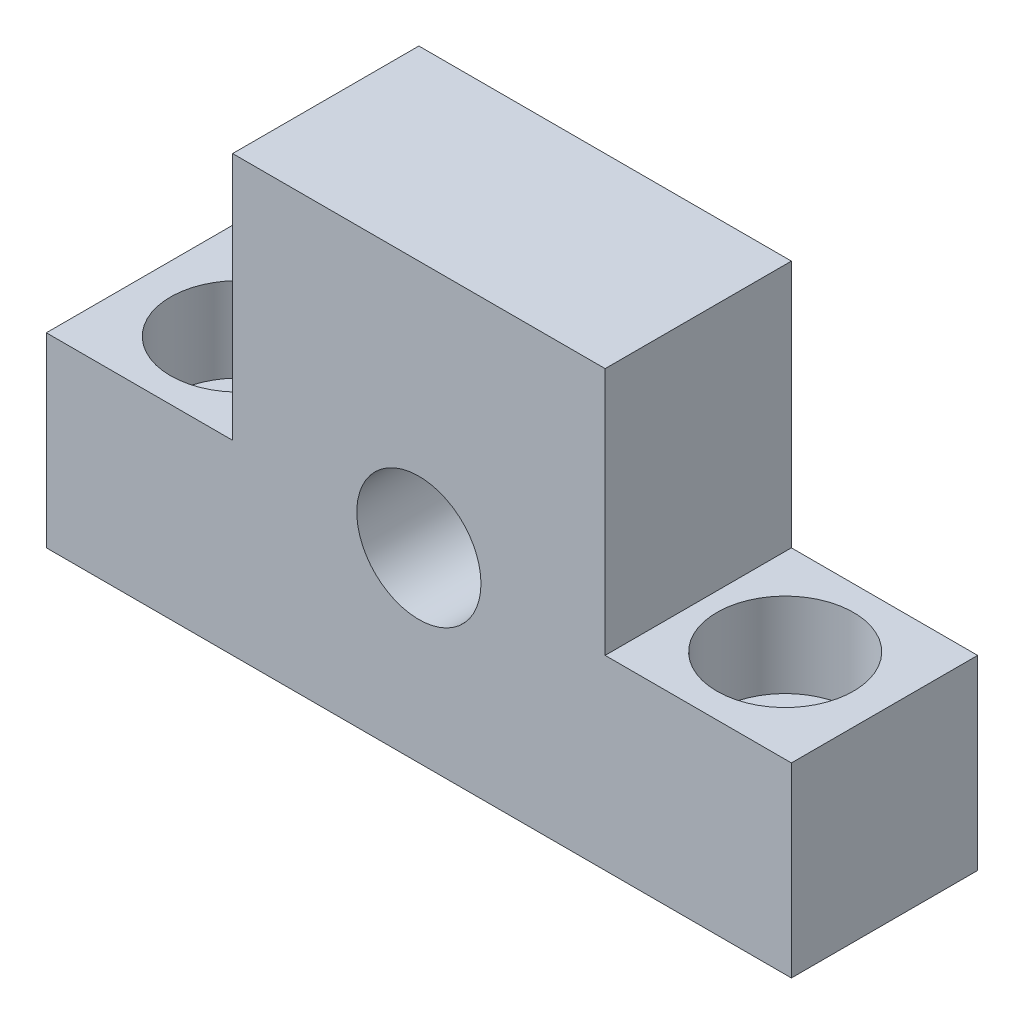
SolidWorks part; units mm, degrees
ref_plane "Front Plane" through (0, 0, 0) normal (0, 0, 1) x (1, 0, 0)
ref_plane "Top Plane" through (0, 0, 0) normal (0, 1, 0) x (1, 0, 0)
ref_plane "Right Plane" through (0, 0, 0) normal (1, 0, 0) x (0, 0, -1)
sketch "Sketch1" plane through (0, 0, 0) normal (0, 0, 1) x (1, 0, 0)
  line L0 (0, 0) -> (0, 15)
  line L1 (0, 15) -> (15, 15)
  line L2 (15, 15) -> (15, 35)
  line L3 (15, 35) -> (45, 35)
  line L5 (45, 15) -> (45, 35)
  line L6 (60, 15) -> (45, 15)
  line L7 (60, 0) -> (60, 15)
  line L8 (60, 0) -> (0, 0)
  dimension "D1" = 20
  dimension "D2" = 15
  dimension "D3" = 20
  dimension "D4" = 30
  dimension "D5" = 15
  dimension "D6" = 15
extrude "Boss-Extrude1" add sketch "Sketch1" along normal blind 15
sketch "Sketch2" plane through (0, 0, 15) normal (0, 0, 1) x (1, 0, 0)
  line L0 (45, 35) -> (15, 35) construction
  line L1 (15, 35) -> (15, 15) construction
  circle A0 centre (30, 15) radius 5
  dimension "D1" = 20
  dimension "D2" = 15
extrude "Cut-Extrude1" cut sketch "Sketch2" against normal through all
sketch "Sketch3" plane through (0, 15, 0) normal (0, 1, 0) x (1, 0, 0)
  line L0 (0, -15) -> (0, 0) construction
  line L1 (0, 0) -> (60, 0) construction
  line L2 (30, 0) -> (30, -10.9189) construction
  circle A0 centre (8, -7.5) radius 5
  circle A2 centre (52, -7.5) radius 5
  dimension "D1" = 8
hole_wizard "CBORE for M6 Hexagon socket head cap screws1" positions "3DSketch1" profile "Sketch4" counterbore size "M6" standard "GB" end condition through all
sketch3d "3DSketch1"
  point P0 (8, 15, 7.5)
  point P3 (52, 15, 7.5)
sketch "Sketch4" plane through (8, 15, 7.5) normal (1, 0, 0) x (0, 0, 1)
  line L0 (0, 0) -> (0, 15)
  line L1 (0, 15) -> (3.3, 15)
  line L3 (3.3, 15) -> (3.3, 6.8)
  line L4 (3.3, 6.8) -> (5.5, 6.8)
  line L5 (5.5, 6.8) -> (5.5, 0)
  line L7 (5.5, 0) -> (0, 0)
  line L11 (0, -6.35) -> (0, 107.95) construction
  dimension "通孔孔直径" = 6.6
  dimension "通孔孔深度" = 15
  dimension "柱形沉头孔直径" = 11
  dimension "柱形沉头孔深度" = 6.8
equation "\"A\"= \"代号代码\""
equation "\"B\"= \"名称代码\""
